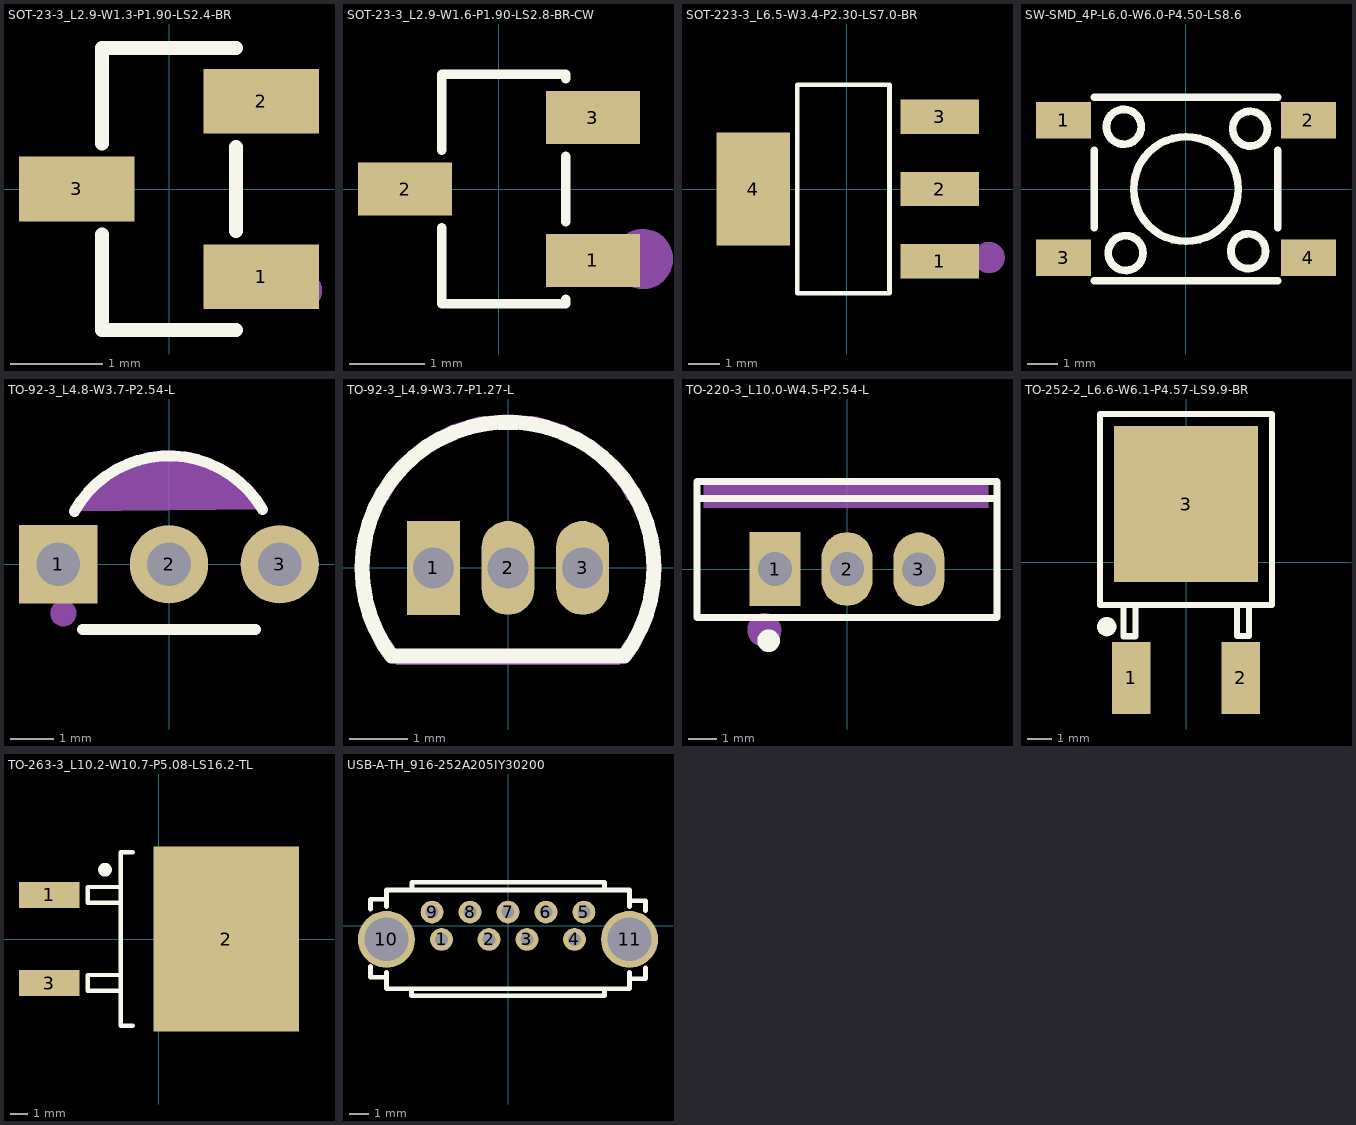
[diagram p0: the footprints below, top view; thin cyan lines are the x and y axes]
# Altium footprint library MISC84402-3.PcbLib: 74 footprints (part 5 of 5)
Each footprint in its own frame and in the unit in brackets; x right, y up, seen from the top. Pads: shape width x height; smd on the part's side, far side on the other; paste and mask are expansions set on the pad; w line width, h text height; cw(c..) or ccw(c..) is an arc to the next point about the centre after c.

## SOT-23-3_L2.9-W1.3-P1.90-LS2.4-BR [mm]
pads (3):
  rect 1.25x0.7 smd: 1(1,-0.95) 2(1,0.95) 3(-1,0)
Top Overlay:
  lines w0.152: -0.726,-0.495 -0.726,-1.526 0.726,-1.526 ; -0.726,0.495 -0.726,1.526 0.726,1.526 ; 0.726,-0.455 0.726,0.455
Mechanical 15:
  circle w0.2: c1.46,-1.1 r0.1

## SOT-23-3_L2.9-W1.6-P1.90-LS2.8-BR-CW [mm]
pads (3):
  rect 1.25x0.7 smd: 1(1.25,-0.95) 2(-1.25,0) 3(1.25,0.95)
Top Overlay:
  lines w0.125: -0.762,-0.517 -0.762,-1.524 0.889,-1.524 0.889,-1.467 ; -0.762,0.517 -0.762,1.524 0.889,1.524 0.889,1.467 ; 0.889,-0.433 0.889,0.433
Mechanical 15:
  circle w0.4: c1.914,-0.931 r0.2

## SOT-223-3_L6.5-W3.4-P2.30-LS7.0-BR [mm]
pads (4):
  rect 2.5x1.1 smd: 1(2.97,-2.3) 2(2.97,0) 3(2.97,2.3)
  rect 2.34x3.6 smd: 4(-2.97,0)
Top Overlay:
  lines w0.152: -1.571,-3.326 -1.571,3.326 1.371,3.326 1.371,-3.326 -1.571,-3.326
Mechanical 15:
  circle w0.5: c4.552,-2.188 r0.25

## SW-SMD_4P-L6.0-W6.0-P4.50-LS8.6 [mm]
pads (4):
  rect 1.8x1.2 smd: 1(-4,2.25) 2(4,2.25) 3(-4,-2.25) 4(4,-2.25)
Top Overlay:
  circle w0.254: c0,0 r1.709
  circle w0.254: c-2.032,2.032 r0.568
  circle w0.254: c-1.971,-2.093 r0.568
  circle w0.254: c2.093,1.971 r0.568
  circle w0.254: c2.032,-2.032 r0.568
  lines w0.254: -3,-3 3,-3 ; -3,-1.269 -3,1.269 ; -3,3 3,3 ; 3,-1.269 3,1.269

## TO-92-3_L4.8-W3.7-P2.54-L [mm]
pads (3):
  rect 1.8x1.8 hole 1: 1(-2.54,0)
  round 1.8 hole 1: 2(0,0) 3(2.54,0)
Top Overlay:
  lines w0.254: -2.171,1.211 cw(c0,0) 2.144,1.26 ; -1.98,-1.5 1.98,-1.5
Mechanical 15:
  circle w0.3: c-2.422,-1.124 r0.15
  region: 2.146,1.261 2.077,1.388 1.767,1.767 1.388,2.078 0.956,2.308 0.487,2.451 0,2.499 -0.487,2.451 -0.956,2.308 -1.388,2.078 -1.767,1.767 -2.077,1.388 -2.172,1.212 -2.171,1.211

## TO-92-3_L4.9-W3.7-P1.27-L [mm]
pads (3):
  rect 0.9x1.6 hole 0.7: 1(-1.27,0)
  oval 0.9x1.6 hole 0.7: 2(0,0) 3(1.27,0)
Top Overlay:
  lines w0.254: -1.981,-1.501 cw(c0,-0.003) 1.981,-1.501 ; -1.98,-1.5 1.98,-1.5
Mechanical 15:
  region: -1.905,-1.397 1.905,-1.397 1.905,-1.651 -1.905,-1.651
  region: -2.29,1.16 -2.036,1.16 -1.926,1.367 -1.638,1.717 -1.288,2.004 -0.888,2.218 -0.455,2.349 -0.004,2.394 0.447,2.349 0.88,2.218 1.28,2.004 1.63,1.717 1.918,1.367 2.028,1.16 2.282,1.16 2.16,1.417 2.127,1.481 1.808,1.869 1.42,2.188 0.977,2.424 0.496,2.57 -0.004,2.619 -0.504,2.57 -0.985,2.424 -1.428,2.188 -1.816,1.869 -2.135,1.481 -2.168,1.417 -2.163,1.414

## TO-220-3_L10.0-W4.5-P2.54-L [mm]
pads (3):
  rect 1.8x2.6 hole 1.2: 1(-2.54,0.005)
  oval 1.8x2.6 hole 1.2: 2(0,0.005) 3(2.54,-0.005)
Top Overlay:
  lines w0.254: -5.3,2.495 5.3,2.495 ; -5.301,-1.704 5.301,-1.704 5.301,3.094 -5.301,3.094 -5.301,3.089 -5.301,-1.704
  lines w0.4: -2.77,-2.33 ccw(c-2.769,-2.53) -2.768,-2.33
Mechanical 15:
  circle w0.6: c-2.921,-2.154 r0.3
  region: -5.06,3.01 -5.06,2.17 4.99,2.17 4.99,3.01

## TO-252-2_L6.6-W6.1-P4.57-LS9.9-BR [mm]
pads (3):
  rect 1.6x3 smd: 1(-2.285,-4.806) 2(2.285,-4.8)
  rect 6x6.5 smd: 3(0,2.428)
Top Overlay:
  lines w0.254: -2.6,-1.771 -2.6,-3.071 -2.1,-3.071 -2.1,-1.771 ; 2.122,-1.767 2.122,-3.067 2.623,-3.067 2.623,-1.767 ; -3.573,-1.771 -3.573,6.179 3.573,6.179 3.573,-1.771 -3.573,-1.771
  lines w0.4: -3.099,-2.674 cw(c-3.299,-2.672) -3.099,-2.671
Mechanical 15:
  circle w0.4: c-2.337,-4.44 r0.2

## TO-263-3_L10.2-W10.7-P5.08-LS16.2-TL [mm]
pads (3):
  rect 3.504x1.5 smd: 1(-6.326,2.54) 3(-6.326,-2.54)
  rect 8.38x10.7 smd: 2(3.888,0)
Top Overlay:
  lines w0.254: -2.213,-2.98 -4.113,-2.98 -4.113,-2.08 -2.213,-2.08 ; -2.213,2.1 -4.113,2.1 -4.113,3 -2.213,3 ; -1.513,-5 -2.213,-5 -2.213,5 -1.513,5
  lines w0.4: -3.115,3.8 cw(c-3.114,4) -3.113,3.8

## USB-A-TH_916-252A205IY30200 [mm]
pads (11):
  round 1.2 hole 0.7: 1(-3.5,-0.72) 2(-1,-0.72) 3(1,-0.72) 4(3.5,-0.72) 5(4,0.72) 6(2,0.72) 7(0,0.72) 8(-2,0.72) 9(-4,0.72)
  round 3 hole 2.3: 10(-6.4,-0.72) 11(6.4,-0.72)
Top Overlay:
  lines w0.254: -7.239,-2.149 -7.239,-2.709 -6.4,-2.709 ; -7.239,0.879 -7.239,1.397 -6.4,1.397 ; -6.4,-2.451 -6.4,-3.32 6.4,-3.32 6.4,-2.451 ; -6.4,1.011 -6.4,1.88 6.4,1.88 6.4,1.011 ; -5.08,-3.32 -5.08,-3.683 5.08,-3.683 5.08,-3.32 ; -5.055,1.88 -5.055,2.286 5.08,2.286 5.08,1.88 ; 6.4,-2.794 7.239,-2.794 7.239,-2.234 ; 6.4,1.312 7.239,1.312 7.239,0.794